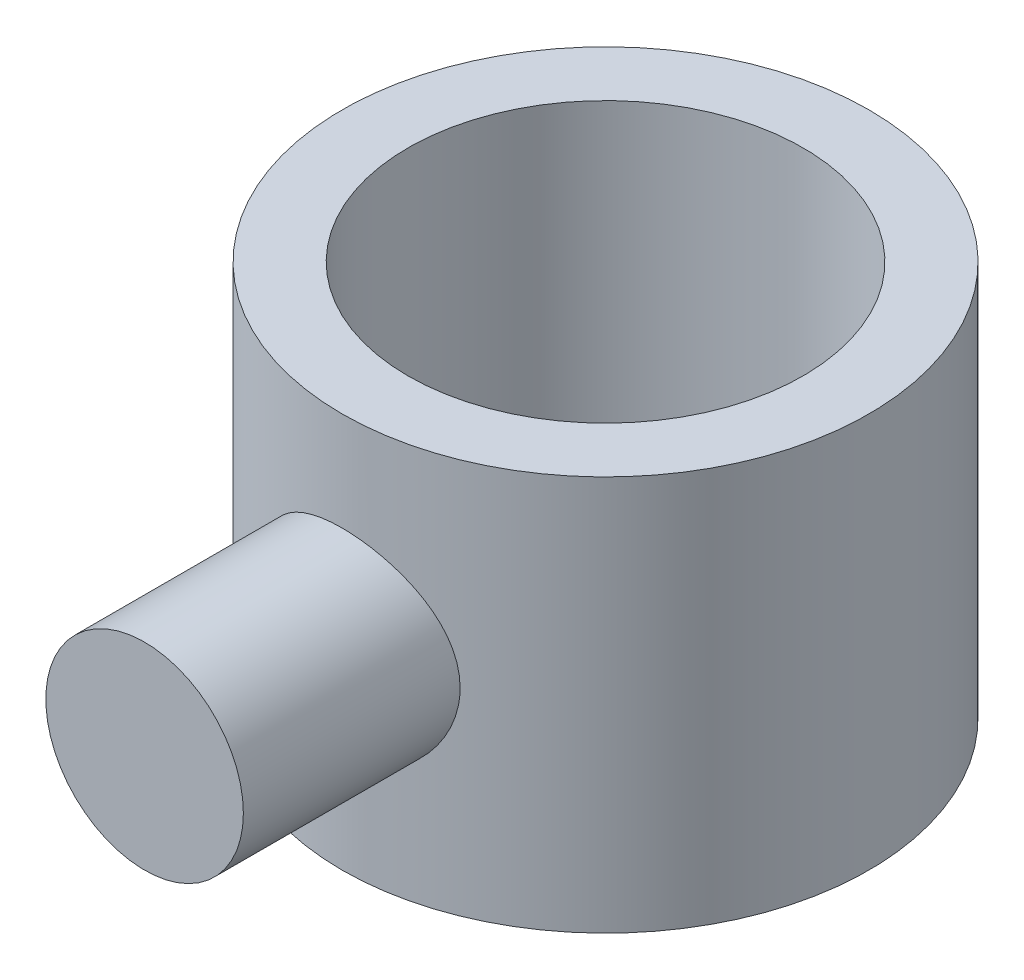
SolidWorks part; units mm, degrees
ref_plane "Front Plane" through (0, 0, 0) normal (0, 0, 1) x (1, 0, 0)
ref_plane "Top Plane" through (0, 0, 0) normal (0, 1, 0) x (1, 0, 0)
ref_plane "Right Plane" through (0, 0, 0) normal (1, 0, 0) x (0, 0, -1)
other "Configuration Table"
sketch "Sketch1" plane through (0, 0, 0) normal (0, 1, 0) x (1, 0, 0)
  circle A0 centre (0, 0) radius 3
  circle A1 centre (0, 0) radius 4
  dimension "D1" = 6
  dimension "D2" = 8
extrude "Boss-Extrude1" add sketch "Sketch1" along normal blind 6
ref_plane "Plane1" through (0, 0, 7) normal (0, 0, 1) x (1, 0, 0)
sketch "Sketch2" plane through (0, 0, 7) normal (0, 0, 1) x (1, 0, 0)
  circle A0 centre (0, 3) radius 1.5
  dimension "D1" = 3
  dimension "D2" = 3
extrude "Boss-Extrude2" add sketch "Sketch2" against normal up to surface (3.2919 mm away)
